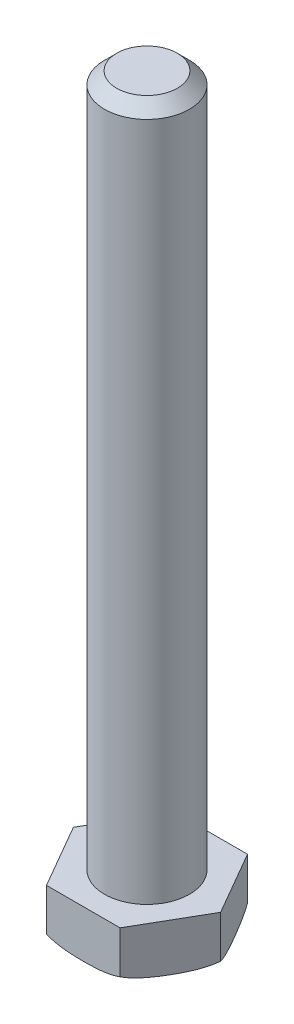
SolidWorks part; units mm, degrees
ref_plane "Front" through (0, 0, 0) normal (0, 0, 1) x (1, 0, 0)
ref_plane "Top" through (0, 0, 0) normal (0, 1, 0) x (1, 0, 0)
ref_plane "Right" through (0, 0, 0) normal (1, 0, 0) x (0, 0, -1)
sketch "Sketch1" plane through (0, 0, 0) normal (0, 1, 0) x (1, 0, 0)
  line L1 (12.1244, 0) -> (6.0622, 10.5)
  line L2 (6.0622, 10.5) -> (-6.0622, 10.5)
  line L3 (-6.0622, 10.5) -> (-12.1244, 0)
  line L4 (-12.1244, 0) -> (-6.0622, -10.5)
  line L5 (-6.0622, -10.5) -> (6.0622, -10.5)
  line L6 (6.0622, -10.5) -> (12.1244, 0)
  circle A0 centre (0, 0) radius 10.5 construction
  dimension "D1" = 21
extrude "Boss-Extrude1" add sketch "Sketch1" along normal blind 8
sketch "Sketch2" plane through (0, 8, 0) normal (0, 1, 0) x (1, 0, 0)
  circle A0 centre (0, 0) radius 7
  dimension "D1" = 14
extrude "Boss-Extrude2" add sketch "Sketch2" along normal blind 114
chamfer "Chamfer1" distance 2 angle 45 1 edges at (0, 122, 7)
sketch "Sketch3" plane through (0, 0, 0) normal (0, 0, 1) x (1, 0, 0)
  line L0 (-12.1244, 0) -> (-12.1244, 1)
  line L1 (-12.1244, 0) -> (-9.1244, 0)
  line L2 (0, 0) -> (0, 6.5979) construction
  arc A0 (-12.1244, 1) -> (-9.1244, 0) centre (-9.1244, 5) ccw
  dimension "D3" = 5
  dimension "D1" = 1
  dimension "D2" = 3
revolve "Cut-Revolve1" cut sketch "Sketch3" angle 360 about L2
scale "Scale 1" bodies to scale 103 scale about centroid uniform scaling yes scale factor 1.875
